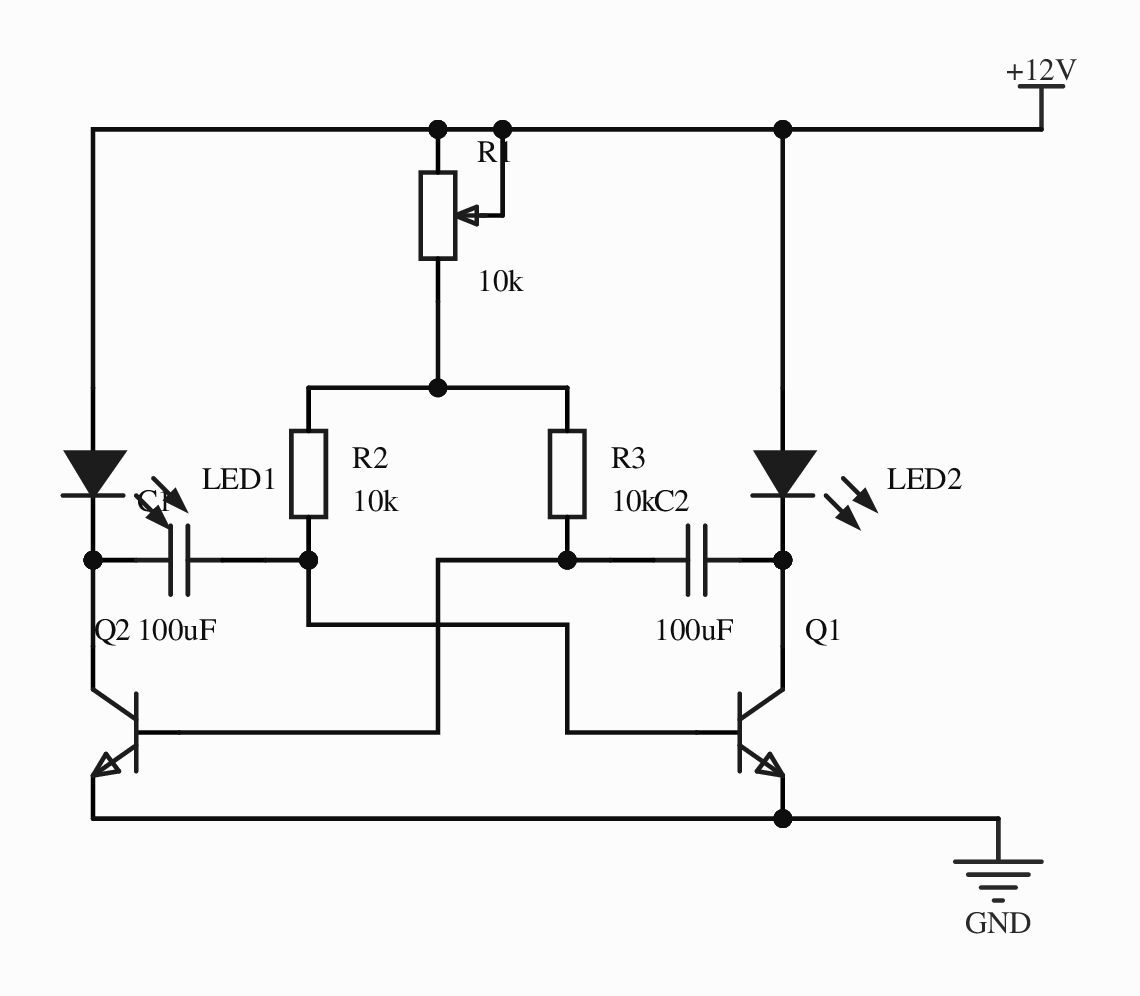
[diagram p0: MISC52066-3.schdoc]
# Altium project MISC52066-2.PrjPcb
1 sheet, 9 parts. Net scope: global (net labels, ports and power ports of the same name join across sheets).
Board file: MISC52066.pcbdoc

## Sheet MISC52066-3.schdoc
size 297 x 209 mm; Version: V1.0; @Project Name: MISC52066; @Update Date: 2026-09-22; @Create Date: 2026-09-22; @Board Name: MISC52066; @Create Time: 19:38:29; @Page Count: 1; @Page No: 1; @Schematic Name: MISC52066; @Update Time: 19:38:29; Size: A4

### Parts
C1  100uF  [CAP-TH_L5.1-W3.2-P5.08-D0.50]
C2  100uF  [CAP-TH_L5.1-W3.2-P5.08-D0.50]
LED1  (no value)  [LED_TH-3mm]
LED2  (no value)  [LED_TH-3mm]
Q1  (no value)  [S8050_TO_92]
Q2  (no value)  [S8050_TO_92]
R1  10k  [R_3296]
R2  10k  [Res_1/8W]
R3  10k  [Res_1/8W]

### Nets
+12V: LED1.1(C) LED2.1(C) R1.2 R1.3
GND: Q1.1(E) Q2.1(E)
NetC1_1: C1.1 LED1.2(A) Q2.3(C)
NetC1_2: C1.2 Q1.2(B) R2.1
NetC2_1: C2.1 LED2.2(A) Q1.3(C)
NetC2_2: C2.2 Q2.2(B) R3.1
NetR1_1: R1.1 R2.2 R3.2

### Library data of the parts
C1 C2 = C323C104K5R5TA7301: 容值:100nF;精度:±10%;额定电压:50V;温度系数:X7R;; Manufacturer: KEMET(基美); AddInBom: yes; ModelId: 5e578892460b443ea6286c5f4e214fbb0819f05c4eef4c71ace90d822a990e87; ModelTransform: 219.6846,125.5903,0,0,0,0,0,0,-196.85; Tolerance: ±10%; Voltage Rating: 50V; Temperature Coefficient: X7R; Pin Spacing: 5.08mm; Symbol: C323C104K5R5TA7301; Device: C323C104K5R5TA7301; Value: 100uF; FootprintName: CAP-TH_L5.1-W3.2-P5.08-D0.50; LCSC Part Name: 100nF ±10% 50V; ManufacturerPart: C323C104K5R5TA7301; Supplier Footprint: 插件,P=5.08mm; JLCPCB Part Class: Extended Part; Datasheet: https://item.szlcsc.com/datasheet/C323C104K5R5TA7301/194969.html; Supplier: LCSC; ConvertToPcb: yes; ModelName: CAP-TH_L5.1-W3.2-P5.08-D0.50
LED1 LED2 = LED_TH-B_3mm: ConvertToPcb: yes; ModelId: ff771fff7070432ca3f353cf0f67af4c0819f05c4eef4c71ace90d822a990e87; ModelName: LED-TH_BD3.8-P2.54-FD_BLUE; ModelTransform: 134.36,149.37,405.47,0,0,0,-11.81,0,-196.85; Symbol: LED_TH-B; Device: LED_TH-B_3mm; FootprintName: LED_TH-3mm; AddInBom: yes; Supplier Footprint: 插件
Q1 Q2 = S8050_TO_NPN: ConvertToPcb: yes; ModelId: aafe8e06f2154e7c93506efd0d6632dd0819f05c4eef4c71ace90d822a990e87; ModelName: TO-92-3_L4.9-W3.7-P1.27-L; ModelTransform: 180.78,141.44,417.3,0,0,0,0,0,-200; Symbol: S8050_TO_NPN; Device: S8050_TO_NPN; FootprintName: S8050_TO_92; AddInBom: yes; Supplier Footprint: TO-92
R1 = R_3296: ConvertToPcb: yes; ModelId: b182808559bb43bda9e7de64b64134cb0819f05c4eef4c71ace90d822a990e87; ModelName: 3296W; ModelTransform: 373.98,188.96,590.49,180,0,0,0,0,-140; Symbol: R_3296; Device: R_3296; Value: 10k; FootprintName: R_3296; AddInBom: yes; Supplier Footprint: 直插
R2 R3 = Res_AXIAL-1/8W: Symbol: 电阻; ConvertToPcb: yes; ModelId: b2b5ae7ae4c642178fe0039925c86a3f0819f05c4eef4c71ace90d822a990e87; ModelName: RES-TH_BD1.8-L3.2-P7.20-D0.4; ModelTransform: 282.86,66.88,253.09,0,0,0,0,0,-191; Device: Res_AXIAL-1/8W; Value: 10k; AddInBom: yes; Supplier Footprint: 轴向引线; FootprintName: Res_1/8W